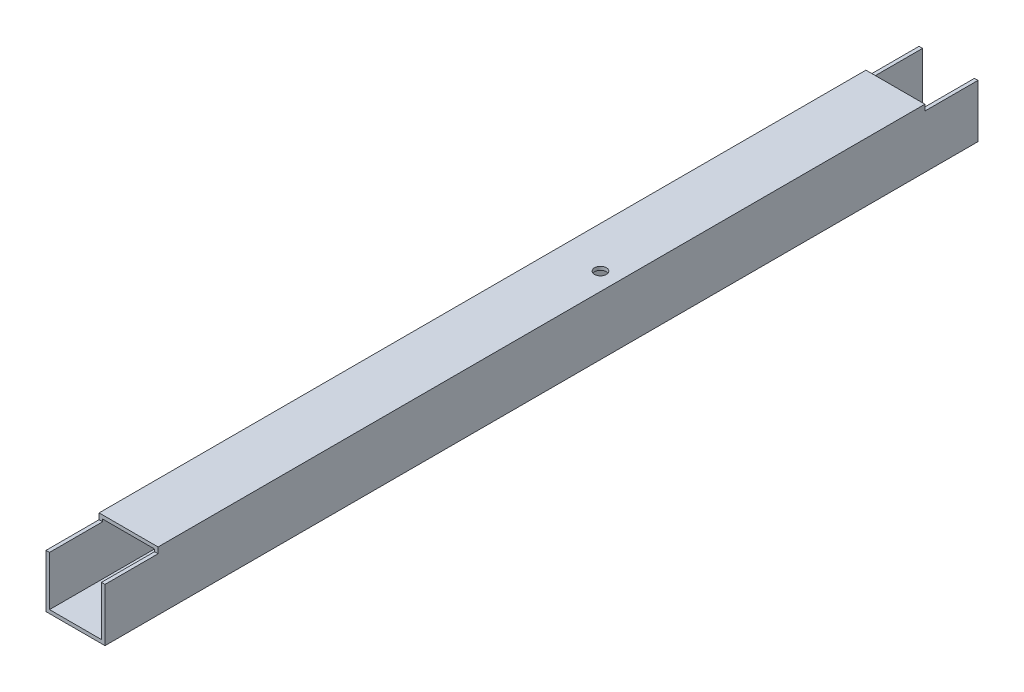
SolidWorks part; units mm, degrees
ref_plane "前视基准面" through (0, 0, 0) normal (0, 0, 1) x (1, 0, 0)
ref_plane "上视基准面" through (0, 0, 0) normal (0, 1, 0) x (1, 0, 0)
ref_plane "右视基准面" through (0, 0, 0) normal (1, 0, 0) x (0, 0, -1)
sketch "草图1" plane through (0, 0, 0) normal (0, 0, 1) x (1, 0, 0)
  line L0 (0, 0) -> (0, 50)
  line L1 (0, 50) -> (50, 50)
  line L2 (50, 50) -> (50, 0)
  line L3 (50, 0) -> (0, 0)
  line L4 (3, 3) -> (3, 47)
  line L5 (3, 47) -> (47, 47)
  line L6 (47, 47) -> (47, 3)
  line L7 (47, 3) -> (3, 3)
  dimension "D1" = 3
extrude "凸台-拉伸1" add sketch "草图1" along normal blind 790
sketch "草图2" plane through (0, 50, 0) normal (0, 1, 0) x (1, 0, 0)
  line L0 (0, 0) -> (0, -45)
  line L1 (0, -790) -> (0, 0) construction
  line L2 (0, -45) -> (50, -45)
  line L3 (50, -790) -> (50, 0) construction
  line L4 (50, -45) -> (50, 0)
  line L5 (50, 0) -> (0, 0)
  line L6 (0, -790) -> (0, -745)
  line L7 (0, -745) -> (50, -745)
  line L8 (50, -745) -> (50, -790)
  line L9 (50, -790) -> (0, -790)
extrude "切除-拉伸1" cut sketch "草图2" against normal blind 5
sketch "草图3" plane through (0, 50, 0) normal (0, 1, 0) x (1, 0, 0)
  line L0 (50, -45) -> (50, -330)
  line L1 (50, -745) -> (50, -45) construction
  line L2 (50, -330) -> (35, -330)
  circle A0 centre (35, -330) radius 5
extrude "切除-拉伸2" cut sketch "草图3" against normal blind 5
sketch "草图4" plane through (0, 0, 790) normal (0, 0, 1) x (1, 0, 0)
  line L16 (50, 0) -> (50, 45)
  line L17 (50, 45) -> (47, 45)
  line L18 (47, 45) -> (47, 3)
  line L19 (47, 3) -> (3, 3)
  line L20 (3, 3) -> (3, 45)
  line L21 (3, 45) -> (0, 45)
  line L22 (0, 45) -> (0, 0)
  line L23 (0, 0) -> (50, 0)
  line L24 (50, 0) -> (50, 45)
  line L25 (50, 45) -> (47, 45)
  line L26 (47, 45) -> (47, 3)
  line L27 (47, 3) -> (3, 3)
  line L28 (3, 3) -> (3, 45)
  line L29 (3, 45) -> (0, 45)
  line L30 (0, 45) -> (0, 0)
  line L31 (0, 0) -> (50, 0)
  dimension "D1" = 0
extrude "切除-拉伸3" cut sketch "草图4" against normal blind 50
sketch "草图5" plane through (0, 0, 745) normal (0, 0, 1) x (1, 0, 0)
  line L16 (47, 47) -> (47, 45)
  line L17 (47, 45) -> (50, 45)
  line L18 (50, 45) -> (50, 50)
  line L19 (50, 50) -> (0, 50)
  line L20 (0, 50) -> (0, 45)
  line L21 (0, 45) -> (3, 45)
  line L22 (3, 45) -> (3, 47)
  line L23 (3, 47) -> (47, 47)
  line L24 (47, 47) -> (47, 45)
  line L25 (47, 45) -> (50, 45)
  line L26 (50, 45) -> (50, 50)
  line L27 (50, 50) -> (0, 50)
  line L28 (0, 50) -> (0, 45)
  line L29 (0, 45) -> (3, 45)
  line L30 (3, 45) -> (3, 47)
  line L31 (3, 47) -> (47, 47)
  dimension "D1" = 0
extrude "切除-拉伸4" cut sketch "草图5" against normal blind 50
sketch "草图6" plane through (0, 0, 695) normal (0, 0, 1) x (1, 0, 0)
  line L16 (3, 47) -> (47, 47)
  line L17 (47, 47) -> (47, 45)
  line L18 (47, 45) -> (50, 45)
  line L19 (50, 45) -> (50, 50)
  line L20 (50, 50) -> (0, 50)
  line L21 (0, 50) -> (0, 45)
  line L22 (0, 45) -> (3, 45)
  line L23 (3, 45) -> (3, 47)
  line L24 (3, 47) -> (47, 47)
  line L25 (47, 47) -> (47, 45)
  line L26 (47, 45) -> (50, 45)
  line L27 (50, 45) -> (50, 50)
  line L28 (50, 50) -> (0, 50)
  line L29 (0, 50) -> (0, 45)
  line L30 (0, 45) -> (3, 45)
  line L31 (3, 45) -> (3, 47)
  dimension "D1" = 0
extrude "凸台-拉伸2" add sketch "草图6" along normal blind 25
sketch "草图7" plane through (0, 0, 740) normal (0, 0, 1) x (1, 0, 0)
  line L16 (0, 0) -> (50, 0)
  line L17 (50, 0) -> (50, 45)
  line L18 (50, 45) -> (47, 45)
  line L19 (47, 45) -> (47, 3)
  line L20 (47, 3) -> (3, 3)
  line L21 (3, 3) -> (3, 45)
  line L22 (3, 45) -> (0, 45)
  line L23 (0, 45) -> (0, 0)
  line L24 (0, 0) -> (50, 0)
  line L25 (50, 0) -> (50, 45)
  line L26 (50, 45) -> (47, 45)
  line L27 (47, 45) -> (47, 3)
  line L28 (47, 3) -> (3, 3)
  line L29 (3, 3) -> (3, 45)
  line L30 (3, 45) -> (0, 45)
  line L31 (0, 45) -> (0, 0)
  dimension "D1" = 0
extrude "凸台-拉伸3" add sketch "草图7" along normal blind 25
sketch "草图8" plane through (0, 0, 0) normal (0, 0, -1) x (-1, 0, 0)
  line L16 (0, 0) -> (0, 45)
  line L17 (0, 45) -> (-3, 45)
  line L18 (-3, 45) -> (-3, 3)
  line L19 (-3, 3) -> (-47, 3)
  line L20 (-47, 3) -> (-47, 45)
  line L21 (-47, 45) -> (-50, 45)
  line L22 (-50, 45) -> (-50, 0)
  line L23 (-50, 0) -> (0, 0)
  line L24 (0, 0) -> (0, 45)
  line L25 (0, 45) -> (-3, 45)
  line L26 (-3, 45) -> (-3, 3)
  line L27 (-3, 3) -> (-47, 3)
  line L28 (-47, 3) -> (-47, 45)
  line L29 (-47, 45) -> (-50, 45)
  line L30 (-50, 45) -> (-50, 0)
  line L31 (-50, 0) -> (0, 0)
  dimension "D1" = 0
extrude "切除-拉伸5" cut sketch "草图8" against normal blind 25
sketch "草图9" plane through (0, 0, 45) normal (0, 0, -1) x (-1, 0, 0)
  line L16 (-47, 45) -> (-47, 47)
  line L17 (-47, 47) -> (-3, 47)
  line L18 (-3, 47) -> (-3, 45)
  line L19 (-3, 45) -> (0, 45)
  line L20 (0, 45) -> (0, 50)
  line L21 (0, 50) -> (-50, 50)
  line L22 (-50, 50) -> (-50, 45)
  line L23 (-50, 45) -> (-47, 45)
  line L24 (-47, 45) -> (-47, 47)
  line L25 (-47, 47) -> (-3, 47)
  line L26 (-3, 47) -> (-3, 45)
  line L27 (-3, 45) -> (0, 45)
  line L28 (0, 45) -> (0, 50)
  line L29 (0, 50) -> (-50, 50)
  line L30 (-50, 50) -> (-50, 45)
  line L31 (-50, 45) -> (-47, 45)
  dimension "D1" = 0
extrude "切除-拉伸6" cut sketch "草图9" against normal blind 25
sketch "草图10" plane through (0, 50, 0) normal (0, 1, 0) x (1, 0, 0)
  circle A0 centre (35, -330) radius 5
extrude "切除-拉伸7" cut sketch "草图10" against normal blind 94
